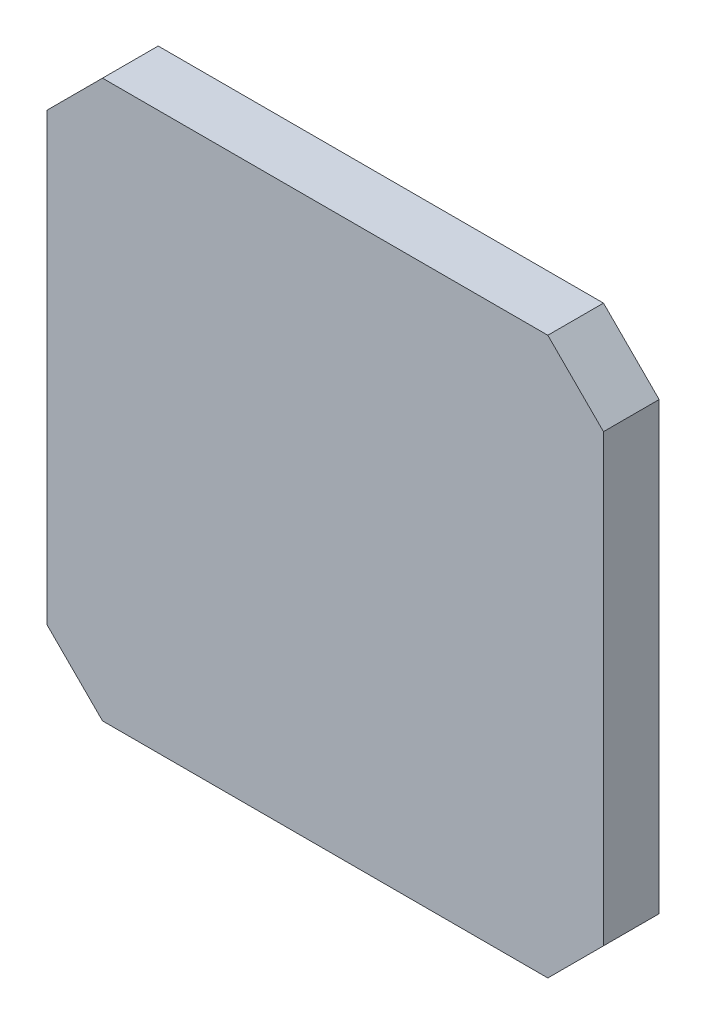
from build123d import *

# Parameters (mm, degrees)
SKETCH1_W           = 50
SKETCH1_H           = 50
BOSS_EXTRUDE1_DEPTH = 5
CHAMFER1_SIZE       = 5


with BuildPart() as part:
    # Sketch1 → Boss-Extrude1 (new body)
    with BuildSketch(Plane.XY):
        with Locations((0.541184779, 3.419811321)):
            Rectangle(SKETCH1_W, SKETCH1_H)
    extrude(amount=BOSS_EXTRUDE1_DEPTH)

    # Chamfer1
    chamfer1_edges = [part.edges().sort_by_distance(p)[0] for p in [
        (-24.458815221, 28.419811321, 2.5),
        (25.541184779, 28.419811321, 2.5),
        (25.541184779, -21.580188679, 2.5),
        (-24.458815221, -21.580188679, 2.5),
    ]]
    chamfer(chamfer1_edges, length=CHAMFER1_SIZE)


solid = part.part
